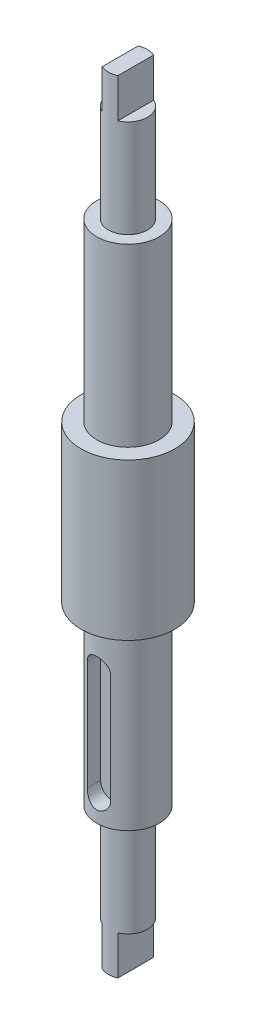
SolidWorks part; units mm, degrees
ref_plane "Front Plane" through (0, 0, 0) normal (0, 0, 1) x (1, 0, 0)
ref_plane "Top Plane" through (0, 0, 0) normal (0, 1, 0) x (1, 0, 0)
ref_plane "Right Plane" through (0, 0, 0) normal (1, 0, 0) x (0, 0, -1)
other "Configuration Table"
sketch "Sketch1" plane through (0, 0, 0) normal (0, 1, 0) x (1, 0, 0)
  circle A0 centre (0, 0) radius 6
  dimension "D1" = 12
extrude "Boss-Extrude1" add sketch "Sketch1" along normal mid plane 20
sketch "Sketch2" plane through (0, 10, 0) normal (0, 1, 0) x (1, 0, 0)
  circle A0 centre (0, 0) radius 4
  dimension "D1" = 8
extrude "Boss-Extrude2" add sketch "Sketch2" along normal blind 22.5
sketch "Sketch3" plane through (0, 32.5, 0) normal (0, 1, 0) x (1, 0, 0)
  circle A0 centre (0, 0) radius 2.5
  dimension "D1" = 5
extrude "Boss-Extrude3" add sketch "Sketch3" along normal blind 12.5
sketch "Sketch4" plane through (0, -10, 0) normal (0, -1, 0) x (1, 0, 0)
  circle A0 centre (0, 0) radius 4
  dimension "D1" = 8
extrude "Boss-Extrude4" add sketch "Sketch4" along normal blind 22.5
sketch "Sketch5" plane through (0, -32.5, 0) normal (0, -1, 0) x (1, 0, 0)
  circle A0 centre (0, 0) radius 2.5
  dimension "D1" = 5
extrude "Boss-Extrude5" add sketch "Sketch5" along normal blind 12.5
sketch "Sketch6" plane through (0, -45, 0) normal (0, -1, 0) x (-1, 0, 0)
  line L0 (1, -2.2913) -> (1, 2.2913)
  line L1 (-1, -2.2913) -> (-1, 2.2913)
  arc A0 (1, 2.2913) -> (-1, 2.2913) centre (0, 0) ccw
  arc A1 (-1, -2.2913) -> (1, -2.2913) centre (0, 0) ccw
  dimension "D3" = 2.5
  dimension "D1" = 2
  dimension "D2" = 1
extrude "Boss-Extrude6" add sketch "Sketch6" along normal blind 5
sketch "Sketch7" plane through (0, 45, 0) normal (0, 1, 0) x (1, 0, 0)
  line L0 (-1, 2.2913) -> (-1, -2.2913)
  line L1 (1, 2.2913) -> (1, -2.2913)
  arc A0 (-1, -2.2913) -> (1, -2.2913) centre (0, 0) ccw
  arc A1 (1, 2.2913) -> (-1, 2.2913) centre (0, 0) ccw
  dimension "D3" = 5
  dimension "D1" = 1
  dimension "D2" = 1
extrude "Boss-Extrude7" add sketch "Sketch7" along normal blind 5
ref_plane "Plane1" through (0, 0, 4) normal (0, 0, 1) x (1, 0, 0)
sketch "Sketch8" plane through (0, 0, 4) normal (0, 0, 1) x (1, 0, 0)
  line L0 (0, 50) -> (0, -50.7758) construction
  line L5 (1, 50) -> (-1, 50) construction
  line L7 (0, -29.5) -> (0, -15.5) construction
  line L8 (-1.5, -29.5) -> (-1.5, -15.5)
  line L9 (1.5, -29.5) -> (1.5, -15.5)
  line L10 (-4, -32.5) -> (4, -32.5) construction
  arc A2 (-1.5, -29.5) -> (1.5, -29.5) centre (0, -29.5) ccw
  arc A3 (1.5, -15.5) -> (-1.5, -15.5) centre (0, -15.5) ccw
  point P2 (0, -22.5)
  dimension "D1" = 3
  dimension "D2" = 14
  dimension "D3" = 10
extrude "Cut-Extrude1" cut sketch "Sketch8" against normal blind 2
